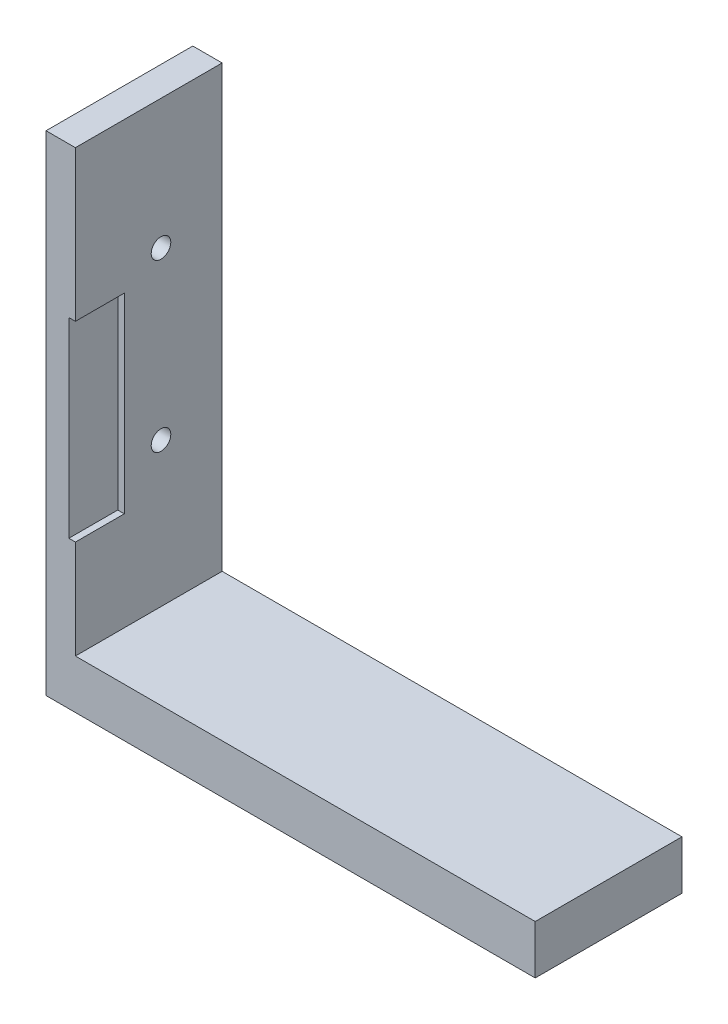
SolidWorks part; units mm, degrees
ref_plane "Front Plane" through (0, 0, 0) normal (0, 0, 1) x (1, 0, 0)
ref_plane "Top Plane" through (0, 0, 0) normal (0, 1, 0) x (1, 0, 0)
ref_plane "Right Plane" through (0, 0, 0) normal (1, 0, 0) x (0, 0, -1)
sketch "Sketch1" plane through (0, 0, 0) normal (0, 0, 1) x (1, 0, 0)
  line L0 (0, 0) -> (100, 0)
  line L1 (0, 0) -> (0, 100)
  line L2 (100, 0) -> (100, 10)
  line L3 (100, 10) -> (6, 10)
  line L4 (6, 10) -> (6, 100)
  line L5 (6, 100) -> (0, 100)
  dimension "D1" = 100
  dimension "D2" = 100
  dimension "D3" = 10
  dimension "D4" = 6
extrude "Boss-Extrude1" add sketch "Sketch1" along normal blind 30
sketch "Sketch2" plane through (0, 0, 0) normal (-1, 0, 0) x (0, 0, 1)
  line L0 (0, 100) -> (0, 0) construction
  line L1 (30, 0) -> (0, 0) construction
  circle A0 centre (12.5, 73.5) radius 2
  circle A1 centre (12.5, 39.5) radius 2
  dimension "D1" = 4
  dimension "D2" = 4
  dimension "D3" = 34
  dimension "D4" = 12.5
  dimension "D5" = 39.5
extrude "Cut-Extrude1" cut sketch "Sketch2" against normal through all
chamfer "Chamfer1" distance 2.1 angle 45 2 edges at (0, 39.5, 14.5) (0, 73.5, 14.5)
sketch "Sketch3" plane through (0, 0, 30) normal (0, 0, 1) x (1, 0, 0)
  line L0 (6, 10) -> (6, 100) construction
  line L1 (7.3391, 69.254) -> (4.6609, 69.254)
  line L2 (7.3391, 69.254) -> (7.3391, 30.178)
  line L3 (7.3391, 30.178) -> (4.6609, 30.178)
  line L4 (4.6609, 69.254) -> (4.6609, 30.178)
  line L5 (7.3391, 69.254) -> (4.6609, 30.178) construction
  line L6 (7.3391, 30.178) -> (4.6609, 69.254) construction
  point P0 (6, 49.716)
extrude "Cut-Extrude2" cut sketch "Sketch3" against normal blind 10
